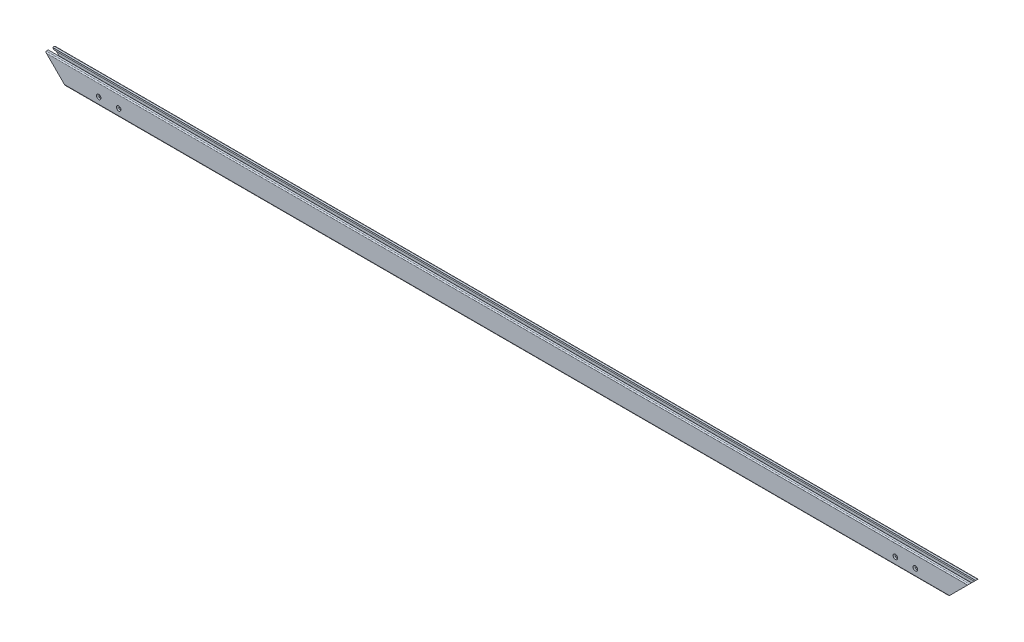
from build123d import *

# Parameters (mm, degrees)
SKETCH11_R          = 2.5
MEMBER_1_DEPTH      = 1386
CUT_EXTRUDE_1_DEPTH = 694.324599304
HOLE_WIZARD_M8_1_D  = 6.8


with BuildPart() as part:
    # Sketch11 → Member 1 (new body)
    with BuildSketch(Plane(origin=(-693, 0, 0), x_dir=(0, 0, -1), z_dir=(1, 0, 0))):
        with BuildLine():
            Line((-6, -15), (-3.25, -15))
            Line((-3.25, -15), (-3.25, -12.7))
            Line((-3.25, -12.7), (-5, -12.7))
            Line((-5, -12.7), (-5, -7))
            ThreePointArc((-5, -7), (0, -4.31662479), (5, -7))
            Line((5, -7), (5, -12.7))
            Line((5, -12.7), (3.25, -12.7))
            Line((3.25, -12.7), (3.25, -15))
            Line((3.25, -15), (6, -15))
            ThreePointArc((6, -15), (7.060660172, -14.560660172), (7.5, -13.5))
            Line((7.5, -13.5), (7.5, 13.5))
            ThreePointArc((7.5, 13.5), (7.060660172, 14.560660172), (6, 15))
            Line((6, 15), (3.25, 15))
            Line((3.25, 15), (3.25, 12.7))
            Line((3.25, 12.7), (5, 12.7))
            Line((5, 12.7), (5, 7))
            ThreePointArc((5, 7), (0, 4.31662479), (-5, 7))
            Line((-5, 7), (-5, 12.7))
            Line((-5, 12.7), (-3.25, 12.7))
            Line((-3.25, 12.7), (-3.25, 15))
            Line((-3.25, 15), (-6, 15))
            ThreePointArc((-6, 15), (-7.060660172, 14.560660172), (-7.5, 13.5))
            Line((-7.5, 13.5), (-7.5, -13.5))
            ThreePointArc((-7.5, -13.5), (-7.060660172, -14.560660172), (-6, -15))
        make_face()
        Circle(SKETCH11_R, mode=Mode.SUBTRACT)
    extrude(amount=MEMBER_1_DEPTH)

    # 草图4 → 切除-拉伸1 (cut, through all)
    with BuildSketch(Plane.XY.offset(7.5)):
        Polygon((-693, 15), (-663, -15), (-693, -15), align=None)
        Polygon((693, -15), (693, 15), (663, -15), align=None)
    extrude(amount=-CUT_EXTRUDE_1_DEPTH, mode=Mode.SUBTRACT)

    # M8 螺纹孔1 (through all)
    with Locations(Plane.XY.offset(7.5)):
        with Locations((-613, -4), (-583, -4), (583, -4), (613, -4)):
            Hole(HOLE_WIZARD_M8_1_D / 2)


solid = part.part
